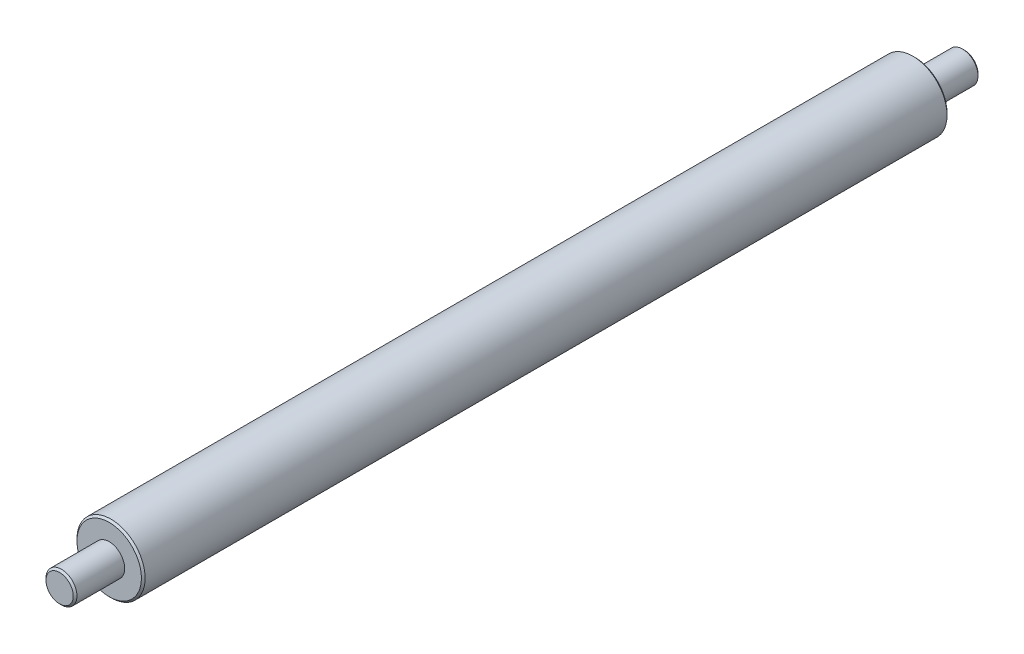
SolidWorks part; units mm, degrees
ref_plane "Front Plane" through (0, 0, 0) normal (0, 0, 1) x (1, 0, 0)
ref_plane "Top Plane" through (0, 0, 0) normal (0, 1, 0) x (1, 0, 0)
ref_plane "Right Plane" through (0, 0, 0) normal (1, 0, 0) x (0, 0, -1)
sketch "Sketch1" plane through (0, 0, 0) normal (0, 0, 1) x (1, 0, 0)
  circle A0 centre (0, 0) radius 27.5
  dimension "D1" = 55
extrude "Boss-Extrude1" add sketch "Sketch1" along normal mid plane 650
sketch "Sketch2" plane through (0, 0, 325) normal (0, 0, 1) x (1, 0, 0)
  circle A0 centre (0, 0) radius 12.5
  dimension "D1" = 25
extrude "Boss-Extrude2" add sketch "Sketch2" along normal blind 40
mirror "Mirror1" about plane through (0, 0, 0) normal (0, 0, 1) of "Boss-Extrude2"
chamfer "Chamfer1" distance 1.5 angle 45 4 edges at (12.5, 0, -365) (27.5, 0, -325) (12.5, 0, 365) (27.5, 0, 325)
